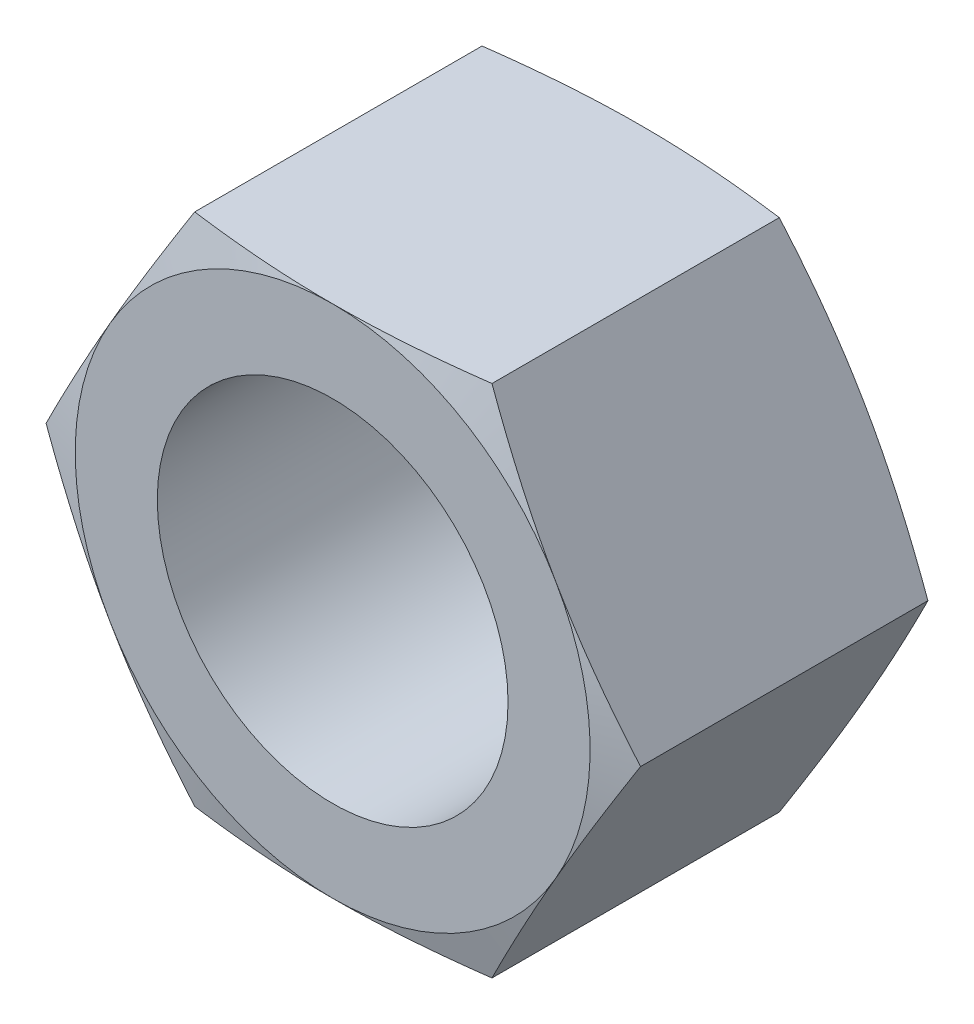
SolidWorks part; units mm, degrees
ref_plane "Plane1" through (0, 0, 0) normal (0, 0, 1) x (1, 0, 0)
ref_plane "Plane2" through (0, 0, 0) normal (0, 1, 0) x (1, 0, 0)
ref_plane "Plane3" through (0, 0, 0) normal (1, 0, 0) x (0, 0, -1)
sketch "dimension sketch" plane through (0, 0, 0) normal (0, 0, 1) x (1, 0, 0)
  line L0 (0, 0) -> (24.1005, 0)
  point P3 (30, 0)
  point P4 (1.5, 0)
  point P5 (50.85, 0)
  point P6 (26.4, 0)
  point P7 (6.4, 0)
  point P8 (46, 0)
sketch "Sketch1" plane through (0, 0, 0) normal (0, 0, 1) x (1, 0, 0)
  line L0 (-26.8088, 0) -> (37.1748, 0) construction
  line L1 (0, 25.0215) -> (0, -25.0215) construction
  line L3 (12.7125, 22.0187) -> (-12.7125, 22.0187)
  line L4 (-12.7125, 22.0187) -> (-25.425, 0)
  line L5 (-25.425, 0) -> (-12.7125, -22.0187)
  line L6 (-12.7125, -22.0187) -> (12.7125, -22.0187)
  line L7 (12.7125, -22.0187) -> (25.425, 0)
  line L8 (25.425, 0) -> (12.7125, 22.0187)
  circle A0 centre (0, 0) radius 22.0187 construction
  circle A1 centre (0, 0) radius 15
extrude "Base-Extrude" add sketch "Sketch1" along normal blind 26.4
cosmetic thread "Cosmetic Thread1" parameters "D2"=31.5
sketch "Sketch2" plane through (0, 0, 0) normal (0, 0, -1) x (-1, 0, 0)
  line L0 (-12.7125, 22.0187) -> (12.7125, 22.0187) construction
  circle A0 centre (0, 0) radius 22.0187
  circle A1 centre (0, 0) radius 15 construction
extrude "Cut-Extrude1" cut sketch "Sketch2" against normal blind 38 draft 75 flip side to cut
sketch "Sketch3" plane through (0, 0, 26.4) normal (0, 0, 1) x (1, 0, 0)
  line L0 (25.425, 0) -> (12.7125, 22.0187) construction
  circle A0 centre (0, 0) radius 22.0187
extrude "Cut-Extrude2" cut sketch "Sketch3" against normal blind 38 draft 75 flip side to cut
chamfer "Chamfer1" [suppressed] distance 0.2 angle 45
equation "\"e@Sketch1\" = \"e@dimension sketch\""
equation "\"D@Sketch1\" = \"D@dimension sketch\""
equation "\"m@Base-Extrude\" = \"m@dimension sketch\""
equation "\"D2@Cosmetic Thread1\" = 1.05 * \"D@dimension sketch\""
